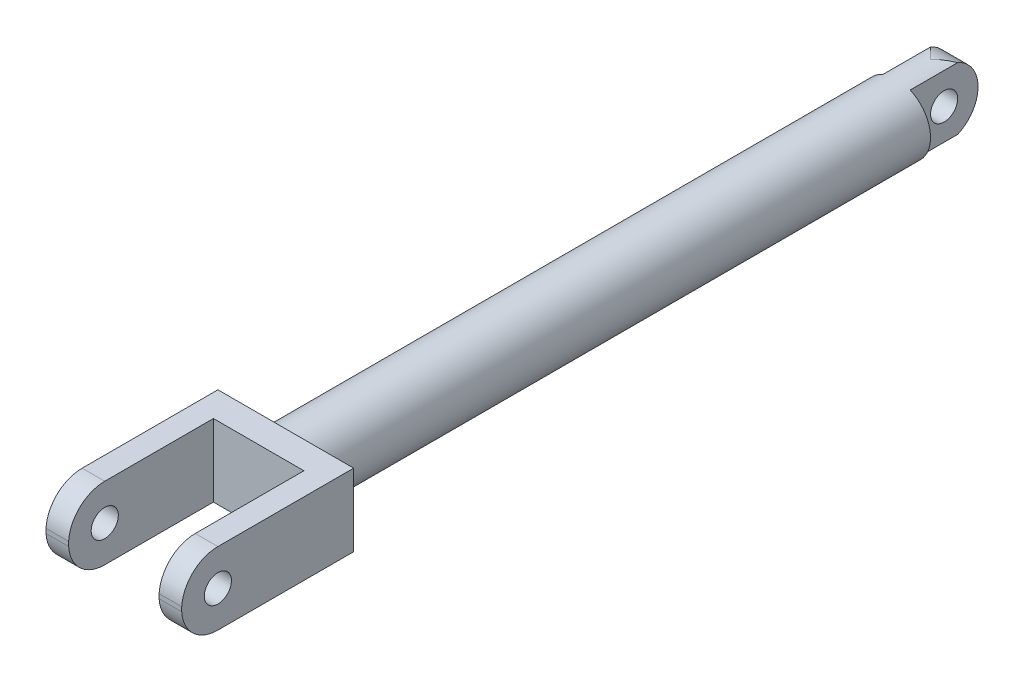
SolidWorks part; units mm, degrees
ref_plane "Front Plane" through (0, 0, 0) normal (0, 0, 1) x (1, 0, 0)
ref_plane "Top Plane" through (0, 0, 0) normal (0, 1, 0) x (1, 0, 0)
ref_plane "Right Plane" through (0, 0, 0) normal (1, 0, 0) x (0, 0, -1)
other "Configuration Table"
sketch "Sketch1" plane through (0, 0, 0) normal (0, 0, 1) x (1, 0, 0)
  circle A0 centre (0, 0) radius 7.5
  dimension "D1" = 15
extrude "Boss-Extrude1" add sketch "Sketch1" along normal blind 150
sketch "Sketch2" plane through (0, 0, 150) normal (0, 0, 1) x (1, 0, 0)
  line L1 (-15, 8) -> (15, 8)
  line L2 (-15, 8) -> (-15, -8)
  line L3 (-15, -8) -> (15, -8)
  line L4 (15, 8) -> (15, -8)
  line L5 (-15, 8) -> (15, -8) construction
  line L6 (-15, -8) -> (15, 8) construction
  point P0 (0, 0)
  dimension "D1" = 30
  dimension "D2" = 16
extrude "Boss-Extrude2" add sketch "Sketch2" along normal blind 38
sketch "Sketch3" plane through (0, 0, 188) normal (0, 0, 1) x (1, 0, 0)
  line L1 (-10, 9.6791) -> (10, 9.6791)
  line L2 (-10, 9.6791) -> (-10, -9.6791)
  line L3 (-10, -9.6791) -> (10, -9.6791)
  line L4 (10, 9.6791) -> (10, -9.6791)
  line L5 (-10, 9.6791) -> (10, -9.6791) construction
  line L6 (-10, -9.6791) -> (10, 9.6791) construction
  point P0 (0, 0)
  dimension "D1" = 20
extrude "Cut-Extrude1" cut sketch "Sketch3" against normal blind 32
sketch "Sketch4" plane through (15, 0, 0) normal (1, 0, 0) x (0, 0, -1)
  line L0 (-180.015, 8) -> (-180.015, 17.7068)
  line L1 (-180.015, 17.7068) -> (-220.3268, 17.7068)
  line L2 (-220.3268, 17.7068) -> (-218.6141, -20.2993)
  line L3 (-218.6141, -20.2993) -> (-180.015, -8)
  circle A0 centre (-180.015, 0) radius 3
  arc A1 (-180.015, 8) -> (-180.015, -8) centre (-180.015, 0) ccw
  dimension "D1" = 6
  dimension "D2" = 16
extrude "Cut-Extrude2" cut sketch "Sketch4" against normal through all both and the other way through all
sketch "Sketch5" plane through (0, 0, 0) normal (0, 1, 0) x (1, 0, 0)
  line L0 (-7.5, 0) -> (-3, 0)
  line L1 (7.5, 0) -> (-7.5, 0) construction
  line L2 (-3, 0) -> (-3, -15)
  line L4 (3, -15) -> (3, 0)
  line L5 (3, 0) -> (22.9427, 0)
  line L6 (22.9427, -15) -> (3, -15)
  line L7 (22.9427, 0) -> (22.9427, -15)
  line L8 (-7.5, 0) -> (-7.5, -15)
  line L9 (-7.5, 0) -> (-7.5, -150) construction
  line L10 (-7.5, -15) -> (-3, -15)
  dimension "D1" = 6
  dimension "D2" = 3
  dimension "D3" = 15
  dimension "D4" = 15
extrude "Cut-Extrude3" cut sketch "Sketch5" against normal through all both and the other way through all
sketch "Sketch6" plane through (-3, 0, 0) normal (-1, 0, 0) x (0, 0, 1)
  line L0 (7.5, 7.5) -> (-1.7271, 19.131)
  line L1 (-1.7271, 19.131) -> (-13.9608, -5.2328)
  line L2 (-13.9608, -5.2328) -> (1.2795, -23.2723)
  line L3 (1.2795, -23.2723) -> (7.5, -7.5)
  line L4 (0, -6.8739) -> (0, 6.8739) construction
  circle A0 centre (7.5, 0) radius 3
  arc A1 (7.5, 7.5) -> (7.5, -7.5) centre (7.5, 0) ccw
  dimension "D1" = 6
extrude "Cut-Extrude4" cut sketch "Sketch6" against normal through all both and the other way through all
